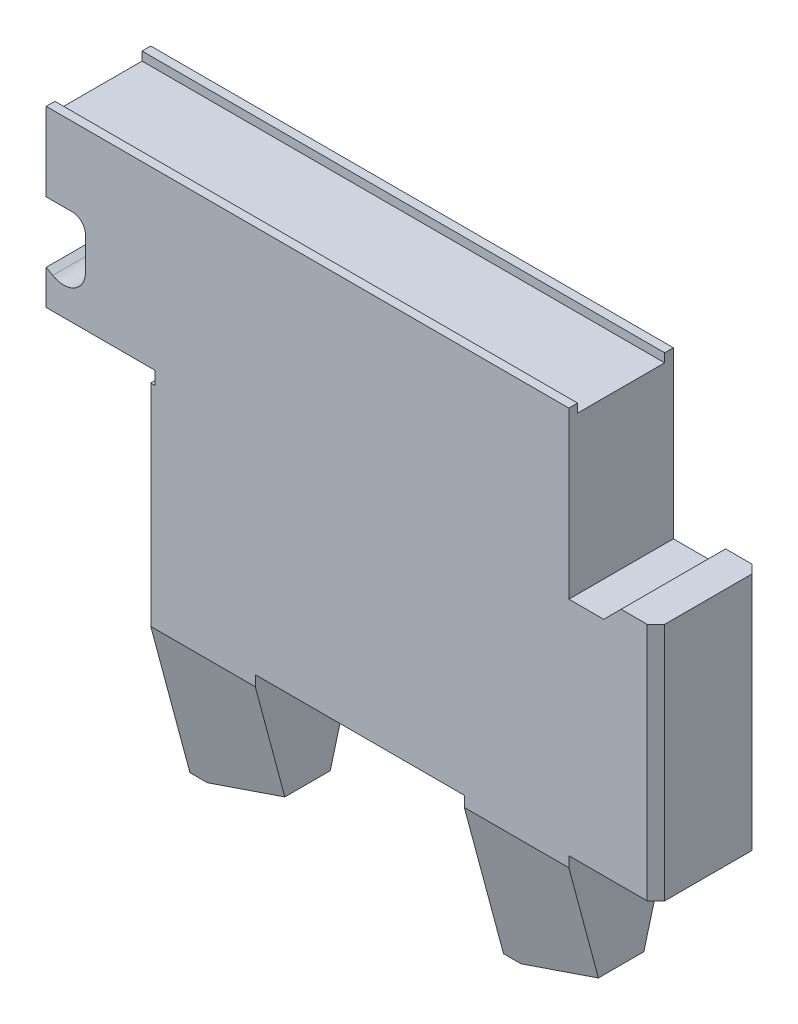
SolidWorks part; units mm, degrees
ref_plane "前视基准面" through (0, 0, 0) normal (0, 0, 1) x (1, 0, 0)
ref_plane "上视基准面" through (0, 0, 0) normal (0, 1, 0) x (1, 0, 0)
ref_plane "右视基准面" through (0, 0, 0) normal (1, 0, 0) x (0, 0, -1)
sketch "草图1" plane through (0, 0, 0) normal (0, 0, 1) x (1, 0, 0)
  line L0 (0, 0) -> (0, 4)
  line L1 (0.75, 3.567) -> (0, 4)
  line L2 (4.5, 5.7321) -> (4.5, 9.5)
  line L3 (3, 11) -> (0, 11)
  line L4 (0, 11) -> (0, 20)
  line L5 (0, 20) -> (60, 20)
  line L6 (60, 20) -> (60, 1)
  line L7 (60, 1) -> (64, 1)
  line L8 (64, 1) -> (66, 3)
  line L9 (66, 3) -> (70, 3)
  line L10 (70, 3) -> (70, -24.5)
  line L11 (70, -24.5) -> (60, -24.5)
  line L12 (60, -38.3579) -> (60, -24.5)
  line L13 (60, -38.3579) -> (50, -42.5)
  line L14 (50, -42.5) -> (48, -42.5)
  line L15 (48, -42.5) -> (48, -24.5)
  line L16 (48, -24.5) -> (24, -24.5)
  line L17 (24, -24.5) -> (24, -38.3579)
  line L18 (24, -38.3579) -> (14, -42.5)
  line L19 (14, -42.5) -> (12, -42.5)
  line L20 (12, -1.5) -> (12, -42.5)
  line L22 (12.5, 0) -> (12.5, -1.5)
  line L23 (12.5, 0) -> (0, 0)
  line L24 (12.5, -1.5) -> (12, -1.5)
  arc A0 (0.75, 3.567) -> (4.5, 5.7321) centre (2, 5.7321) ccw
  arc A1 (4.5, 9.5) -> (3, 11) centre (3, 9.5) ccw
  dimension "D13" = 2.5
  dimension "D15" = 11
  dimension "D1" = 42.5
  dimension "D3" = 1
  dimension "D4" = 4
  dimension "D5" = 45
  dimension "D6" = 2
  dimension "D7" = 22.5
  dimension "D8" = 22.5
  dimension "D9" = 2
  dimension "D10" = 18
  dimension "D11" = 10
  dimension "D12" = 12
  dimension "D14" = 60
  dimension "D16" = 3
  dimension "D17" = 12
  dimension "D18" = 10
  dimension "D19" = 36
  dimension "D20" = 60
  dimension "D21" = 4
  dimension "D22" = 1.5
  dimension "D23" = 0.5
  dimension "D24" = 4.5
  dimension "D25" = 62.5
extrude "凸台-拉伸1" add sketch "草图1" along normal mid plane 12
sketch "草图2" plane through (12, 0, 0) normal (-1, 0, 0) x (0, 0, 1)
  line L0 (0, -42.5) -> (0, -16.2947) construction
  line L1 (6, -25.7058) -> (6, -47.5)
  line L2 (1.5, -42.5) -> (6, -25.7058)
  line L3 (6, -42.5) -> (-6, -42.5) construction
  line L4 (-1.5, -42.5) -> (1.5, -42.5)
  line L5 (-1.5, -42.5) -> (-6, -25.7058)
  line L7 (-6, -1.5) -> (-6, -42.5) construction
  line L8 (-6, -25.7058) -> (-6, -47.5)
  line L9 (-6, -47.5) -> (6, -47.5)
  point P11 (0, -47.5)
  dimension "D1" = 1.5
  dimension "D2" = 75
  dimension "D3" = 5
extrude "切除-拉伸1" cut sketch "草图2" against normal through all
sketch "草图5" plane through (0, 20, 0) normal (0, 1, 0) x (1, 0, 0)
  line L0 (0, -6) -> (0, 6) construction
  line L1 (0, 5) -> (60, 5)
  line L2 (0, 5) -> (0, -5)
  line L3 (0, -5) -> (60, -5)
  line L4 (60, 5) -> (60, -5)
  line L5 (60, -6) -> (60, 6) construction
  dimension "D1" = 10
  dimension "D2" = 5
extrude "切除-拉伸2" cut sketch "草图5" against normal blind 1
chamfer "倒角1" distance 1 angle 45 2 edges at (70, -10.75, -6) (70, -10.75, 6)
